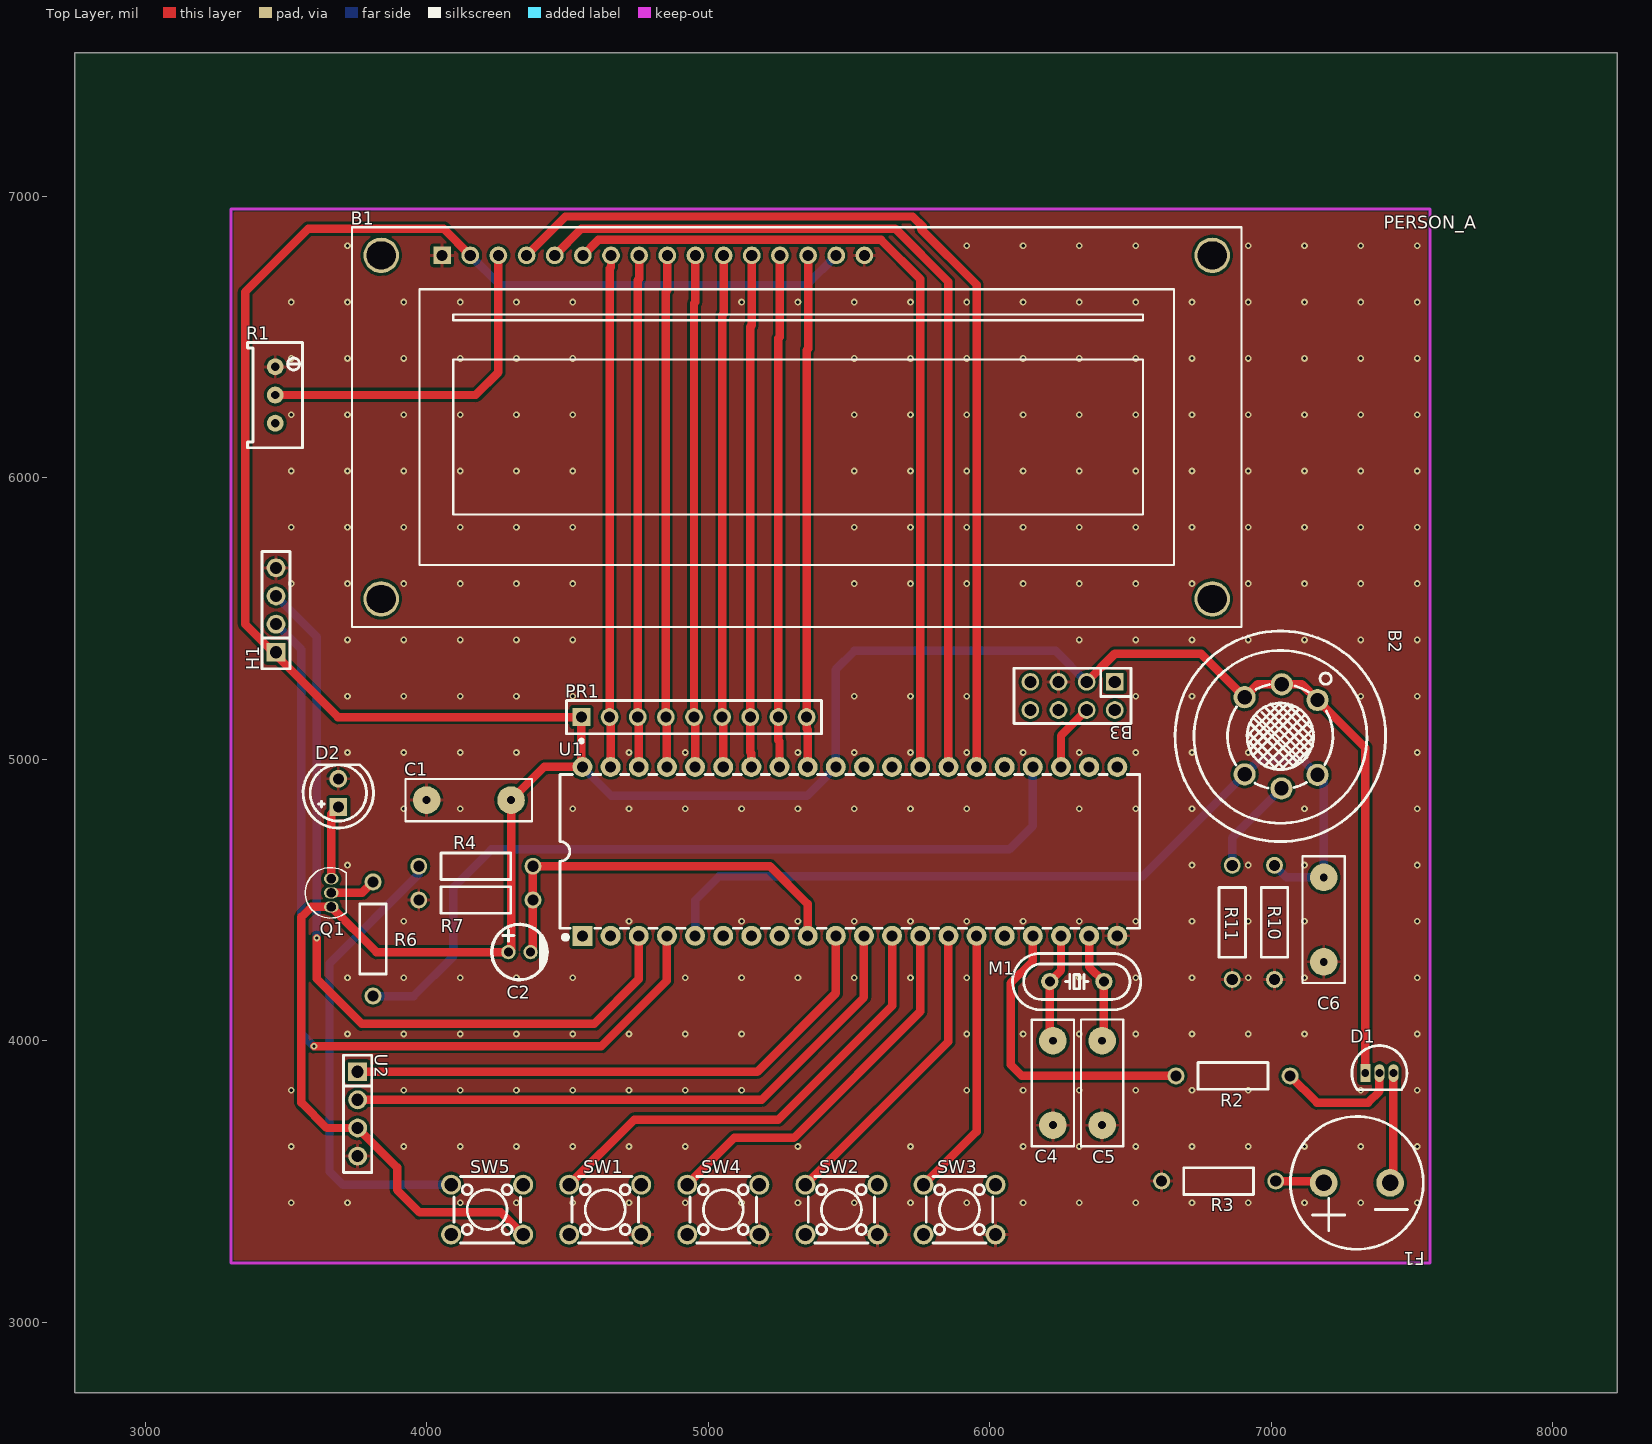
[diagram p0: Top Layer view]
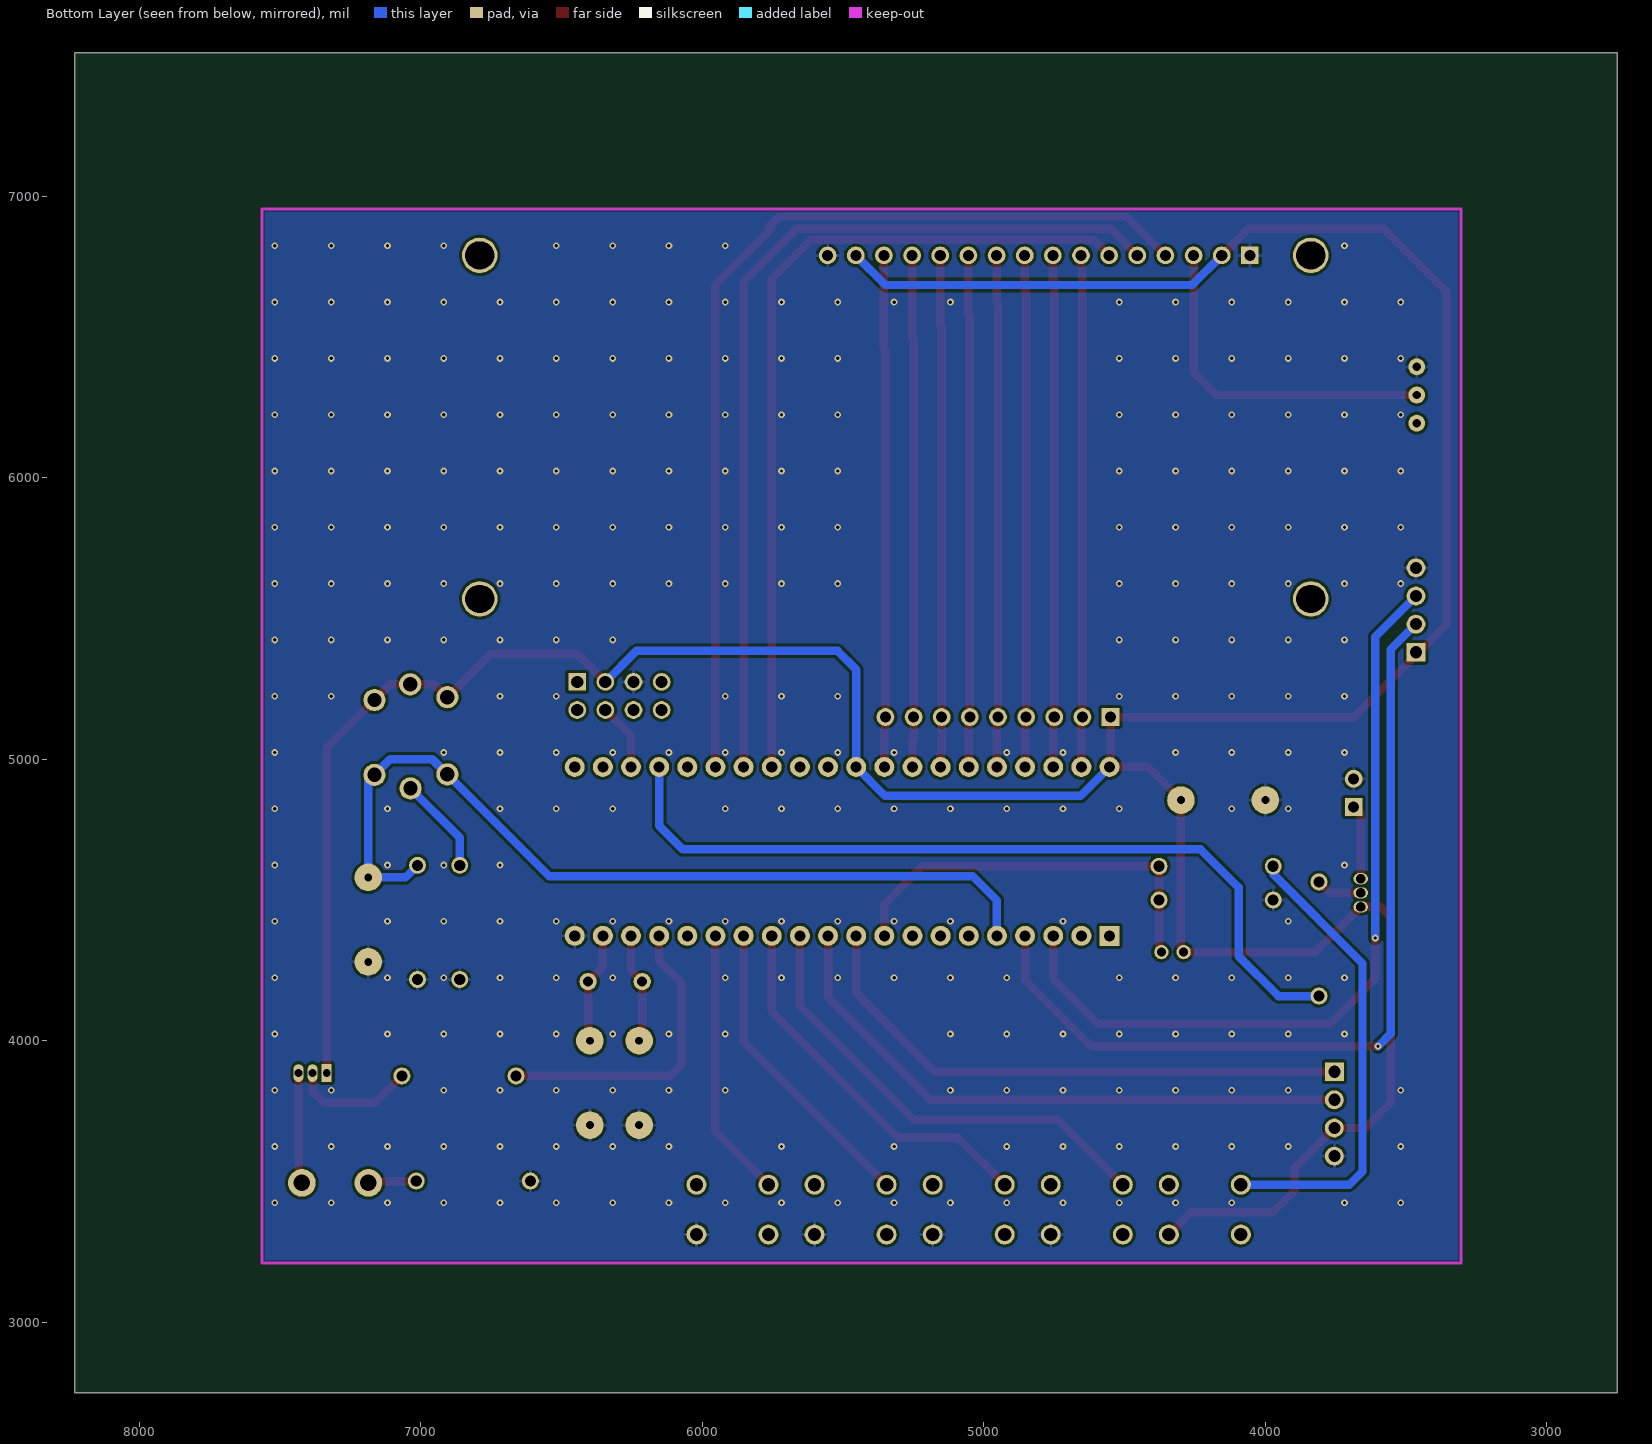
[diagram p1: Bottom Layer view, seen from below]
# Altium PCB MISC75421.pcbdoc
Units mil, origin at the board's own origin, x right, y up, seen from the top; angles counter-clockwise.
Board outline 5480 x 4760 mil, 2 copper layers (Top Layer, Bottom Layer), stack 62.206 mil thick; 30 components, 39 nets, 150 pads, 275 vias.

## Layer stack, top to bottom
Top Solder Mask Layer: solder mask 0.394, Dk 3.3
Top Layer: signal copper 1.379
Dielectric1: surface 59.449, FR4, Dk 4.5
Bottom Layer: signal copper 1.378
Bottom Solder Mask Layer: solder mask 0.394, Dk 3.3

## Board outline
8230,2750 2750,2750 2750,7510 8230,7510

## Design rules (kind name [scope] priority, off if disabled: settings)
BoardOutlineClearance copperThickness2oz_1 [All] p2 off: genericclearance=7.99 ignorepadtopadclearanceinfootprint=FALSE except(0: Arc-SplitContinuation Track-SplitContinuation SMDPad-SplitContinuation THPad-SplitContinuation Via-SplitContinuation Fill-SplitContinuation Region-SplitContinuation Poly-SplitContinuation Text-SplitContinuation Hole-SplitContinuation; 5.98: Arc-CutoutEdge SMDPad-CutoutEdge THPad-CutoutEdge Via-CutoutEdge Fill-CutoutEdge Region-CutoutEdge Text-CutoutEdge; 6.93: Hole-OutlineEdge Hole-CutoutEdge; 10: Poly-OutlineEdge Poly-CutoutEdge; 11.81: Arc-OutlineEdge Track-OutlineEdge SMDPad-OutlineEdge THPad-OutlineEdge Via-OutlineEdge Fill-OutlineEdge Region-OutlineEdge Text-OutlineEdge Track-CutoutEdge)
BoardOutlineClearance copperThickness1oz_1 [All] p4: genericclearance=4.02 ignorepadtopadclearanceinfootprint=FALSE except(0: Arc-SplitContinuation Track-SplitContinuation SMDPad-SplitContinuation THPad-SplitContinuation Via-SplitContinuation Fill-SplitContinuation Region-SplitContinuation Poly-SplitContinuation Text-SplitContinuation Hole-SplitContinuation; 6: SMDPad-CutoutEdge THPad-CutoutEdge Via-CutoutEdge Fill-CutoutEdge Region-CutoutEdge Text-CutoutEdge; 6.93: Hole-OutlineEdge Hole-CutoutEdge; 10: Poly-OutlineEdge Poly-CutoutEdge; 11.8: Arc-OutlineEdge Track-OutlineEdge SMDPad-OutlineEdge THPad-OutlineEdge Via-OutlineEdge Fill-OutlineEdge Region-OutlineEdge Text-OutlineEdge; 11.81: Arc-CutoutEdge Track-CutoutEdge)
Clearance copperThickness2oz [All] p1 off: gap=7.99 ignorepadtopadclearanceinfootprint=FALSE except(5.98: SMDPad-Track SMDPad-SMDPad THPad-Track SMDPad-THPad THPad-THPad Track-Via SMDPad-Via THPad-Via Via-Via Fill-Track Region-Track Fill-SMDPad Region-SMDPad Fill-THPad Region-THPad Fill-Via Region-Via Fill-Fill Fill-Region Region-Region Arc-Track Arc-SMDPad Arc-THPad Arc-Via Fill-Arc Region-Arc Arc-Arc Text-Track SMDPad-Text Text-THPad Text-Via Fill-Text Region-Text Arc-Text Text-Text; 6.93: Hole-Track Hole-SMDPad Hole-THPad Hole-Via Fill-Hole Region-Hole Hole-Arc Hole-Text; 10: Poly-Track Poly-SMDPad Poly-THPad Poly-Via Poly-Fill Poly-Region Poly-Poly Poly-Arc Poly-Text Poly-Hole)
Clearance copperThickness1oz [All] p3: gap=4.02 ignorepadtopadclearanceinfootprint=FALSE except(5.98: SMDPad-Track SMDPad-SMDPad THPad-Track SMDPad-THPad THPad-THPad Track-Via SMDPad-Via THPad-Via Via-Via Fill-Track Region-Track Fill-SMDPad Region-SMDPad Fill-THPad Region-THPad Fill-Via Region-Via Fill-Fill Fill-Region Region-Region; 6: Arc-Track Arc-SMDPad Arc-THPad Arc-Via Fill-Arc Region-Arc Arc-Arc Text-Track SMDPad-Text Text-THPad Text-Via Fill-Text Region-Text Arc-Text Text-Text; 6.93: Hole-Track Hole-SMDPad Hole-THPad Hole-Via Fill-Hole Region-Hole Hole-Arc Hole-Text; 10: Poly-Track Poly-SMDPad Poly-THPad Poly-Via Poly-Fill Poly-Region Poly-Poly Poly-Arc Poly-Text Poly-Hole)
DiffPairsRouting differentialPair [All] p1: maxlimit=6 minlimit=6 mostfreqgap=6 toplayer_minwidth=5 toplayer_prefwidth=10 toplayer_maxwidth=100 toplayer_mingap=6 toplayer_prefgap=6 toplayer_maxgap=6 bottomlayer_minwidth=5 bottomlayer_prefwidth=10 bottomlayer_maxwidth=100 bottomlayer_mingap=6 bottomlayer_prefgap=6 bottomlayer_maxgap=6 maxuncoupledlength=10
HoleToHoleClearance otherClearance [All] p1: gap=11.81 allowstackedmicrovias=TRUE
Length netLength [All] p1: minlimit=0 maxlimit=0
MatchedLengths netLengthTolerance [All] p1: tolerance=1000
PasteMaskExpansion pasteMaskExpansion [All] p1: expansion=0
PlaneConnect innerPlane [All] p1: planeconnectstyle=Relief reliefexpansion=20 reliefentries=4 reliefconductorwidth=10 reliefairgap=10
PolygonConnect copperRegion [(InNet('GND'))] p1: connectstyle=Relief reliefconductorwidth=10 reliefentries=4 polygonreliefangle="90 Angle" airgapwidth=10 via.connectstyle=Relief via.reliefconductorwidth=10 via.reliefentries=4 via.polygonreliefangle="90 Angle" via.airgapwidth=10
RoutingVias viaSize [All] p1: holewidth=12.01 width=24.02 viastyle="Through Hole" minholewidth=11.81 minwidth=19.68 maxholewidth=248.03 maxwidth=393.7
SolderMaskExpansion solderMaskExpansion [IsVia] p1: expansion=-1000 istentingtop=TRUE
SolderMaskExpansion solderMaskExpansion [All] p2: expansion=2 istentingtop=FALSE
Width copperThickness2oz_2 [All] p1 off: maxlimit=100 minlimit=8 preferedwidth=10
Width copperThickness1oz_2 [All] p2: maxlimit=100 minlimit=5 preferedwidth=10

## Components (designator, comment, footprint, x,y, rotation, side; value= is the part's Value field where it differs from the comment)
B1 "LCD1602" LCD1602 5315,6180 r0 top
B2 "MQ-2" SENSOR-TH_MQ-2 7035.68,5081.43 r270 top
B3 "DS18B20U+T&R" HDR-TH_8P-P2.54-V-F-R2-C4-S2.54-1 6295,5225 r180 top
C1 "Cap" RAD-0.3 4150,4855 r0 top
C2 "Electrolytic capacitor" CAP-TH_BD5.0-P2.00-D0.8-FD-10UF50VC110GL 4330,4315 r0 top
C4 "Cap" RAD-0.3 6225,3850 r90 top
C5 "Cap" RAD-0.3 6400,3850 r270 top
C6 "Cap" RAD-0.3 7187.31,4430.37 r270 top
D1 "PNP transistor" S8550P_TO-92 7385,3885 r0 top
D2 "LED0" LED-TH_5mm 3686.26,4880.55 r90 top
F1 "Buzzer" BUZ-TH_BD12.0-P6.00-D0.9-RD 7305,3495 r180 top
H1 "" HDR-TH_4P-P2.54-V-F 3465,5530 r90 top
M1 "Crystal oscillator" HC-49S_L11.5-W5.0-P4.88 6310,4210 r0 top
PR1 "8-resistor 9-pin array" RES-ARRAY-TH_9P-P2.54-D1.0 4950,5150 r0 top
Q1 "PNP" TO-92-3_L4.6-W3.6-P1.27-L_1 3661.26,4525.55 r270 top
R1 "Res Adj2" RES-ADJ-TH_3P-L9.5-W4.85-P2.54_PV36W103C01B00 3462.39,6294.12 r0 top
R2 "?K" Res_1/4W 6865,3875 r0 top
R3 "?K" Res_1/4W 6814.06,3501.48 r180 top
R4 "?K" Res_1/4W 4175,4620 r0 top
R6 "?K" Res_1/4W 3809.62,4361.5 r90 top
R7 "?K" Res_1/4W 4175,4500 r180 top
R10 "?K" Res_1/4W 7012.31,4420.37 r270 top
R11 "?K" Res_1/4W 6862.31,4420.37 r270 top
SW1 "TSW tactile switch" SW-TH_4P-L6.0-W6.0-P4.50-LS6.5 4634.57,3400 r0 top
SW2 "TSW tactile switch" SW-TH_4P-L6.0-W6.0-P4.50-LS6.5 5473.7,3400 r0 top
SW3 "TSW tactile switch" SW-TH_4P-L6.0-W6.0-P4.50-LS6.5 5893.26,3400 r0 top
SW4 "TSW tactile switch" SW-TH_4P-L6.0-W6.0-P4.50-LS6.5 5054.13,3400 r0 top
SW5 "TSW tactile switch" SW-TH_4P-L6.0-W6.0-P4.50-LS6.5 4215,3400 r180 top
U1 "STC12C5A60S2" DIP-40_L52.3-W13.9-P2.54-LS15.2-BL-BASE 5503.78,4672.72 r0 top
U2 "HC05" HDR-TH_4P-P2.54-V-F 3755,3740 r270 top

## Footprints (in the part's own frame and the unit in brackets; to place one, negate y for a bottom-side part, rotate by r counter-clockwise, add the part's x,y. Pads: shape width x height; smd on the part's side, far side on the other; paste and mask are expansions set on the pad)
BUZ-TH_BD12.0-P6.00-D0.9-RD [mm]
  round 2.5 hole 1.5 paste+0 mask+0.05: 1(-3,0) 2(3,0)
  silkscreen extent -5.99,-5.99 5.99,5.99
CAP-TH_BD5.0-P2.00-D0.8-FD-10UF50VC110GL [mm]
  round 1.3 hole 0.8: 1(-1,0) 2(1,0)
  silkscreen extent -2.5,-2.5 2.5,2.5
DIP-40_L52.3-W13.9-P2.54-LS15.2-BL-BASE [mm]
  rect 1.8x1.8 hole 1: 1(-24.13,-7.62)
  round 1.8 hole 1: 2(-21.59,-7.62) 3(-19.05,-7.62) 4(-16.51,-7.62) 5(-13.97,-7.62) 6(-11.43,-7.62) 7(-8.89,-7.62) 8(-6.35,-7.62) 9(-3.81,-7.62) 10(-1.27,-7.62) 11(1.27,-7.62) 12(3.81,-7.62) 13(6.35,-7.62) 14(8.89,-7.62) 15(11.43,-7.62) 16(13.97,-7.62) 17(16.51,-7.62) 18(19.05,-7.62) 19(21.59,-7.62) 20(24.13,-7.62) 21(24.13,7.62) 22(21.59,7.62) 23(19.05,7.62) 24(16.51,7.62) 25(13.97,7.62) 26(11.43,7.62) 27(8.89,7.62) 28(6.35,7.62) 29(3.81,7.62) 30(1.27,7.62) 31(-1.27,7.62) 32(-3.81,7.62) 33(-6.35,7.62) 34(-8.89,7.62) 35(-11.43,7.62) 36(-13.97,7.62) 37(-16.51,7.62) 38(-19.05,7.62) 39(-21.59,7.62) 40(-24.13,7.62)
  silkscreen extent -26.16,-7.95 26.16,6.93
HC-49S_L11.5-W5.0-P4.88 [mm]
  round 1.56 hole 0.9: 1(-2.44,0) 2(2.44,0)
  silkscreen extent -5.8,-2.54 5.77,2.54
HDR-TH_4P-P2.54-V-F [mm]
  rect 1.7x1.7 hole 1.1: 1(-3.81,0)
  round 1.7 hole 1.1: 2(-1.27,0) 3(1.27,0) 4(3.81,0)
  silkscreen extent -5.29,-1.27 5.29,1.27
HDR-TH_8P-P2.54-V-F-R2-C4-S2.54-1 [mm]
  rect 1.6x1.6 hole 1.1: 1(-3.81,-1.27)
  round 1.6 hole 1.1: 2(-3.81,1.27) 3(-1.27,-1.27) 4(-1.27,1.27) 5(1.27,-1.27) 6(1.27,1.27) 7(3.81,-1.27) 8(3.81,1.27)
  silkscreen extent -5.28,-2.5 5.28,2.5
LCD1602 [mm]
  round 3.2 hole 2.5 slot 2.625 at 0 deg: 0(-37.5,-15.5) 0(-37.5,15.5) 0(37.5,-15.5) 0(37.5,15.5)
  rect 1.6x1.6 hole 1: 1(-32,15.5)
  round 1.6 hole 1: 2(-29.46,15.5) 3(-26.92,15.5) 4(-24.38,15.5) 5(-21.84,15.5) 6(-19.3,15.5) 7(-16.76,15.5) 8(-14.22,15.5) 9(-11.68,15.5) 10(-9.14,15.5) 11(-6.6,15.5) 12(-4.06,15.5) 13(-1.52,15.5) 14(1.02,15.5) 15(3.56,15.5) 16(6.1,15.5)
  silkscreen extent -40.13,-18.03 40.13,18.03
LED-TH_5mm [mm]
  rect 1.6x1.6 hole 1 paste+0 mask+0.051: 1(-1.27,0)
  round 1.6 hole 1 paste+0 mask+0.051: 2(1.27,0)
  silkscreen extent -3.17,-3.17 2.54,3.17
RAD-0.3 [mil]
  round 98 hole 28: 1(150,0) 2(-150,0)
  silkscreen extent -225,-75 225,75
RES-ADJ-TH_3P-L9.5-W4.85-P2.54_PV36W103C01B00 [mil]
  round 60 hole 30: 1(0,100) 2(0,0) 3(0,-100)
  silkscreen extent -98,-187 96,187
RES-ARRAY-TH_9P-P2.54-D1.0 [mm]
  rect 1.6x1.6 hole 1: 1(-10.16,0)
  round 1.6 hole 1: 2(-7.62,0) 3(-5.08,0) 4(-2.54,0) 5(0,0) 6(2.54,0) 7(5.08,0) 8(7.62,0) 9(10.16,0)
  silkscreen extent -11.5,-2.31 11.5,1.5
Res_1/4W [mil]
  round 60 hole 39.37 paste+0 mask+2: 1(-202.76,0) 2(202.76,0)
  silkscreen extent -124,-47 124,47
S8550P_TO-92 [mm]
  rect 0.9x1.6 hole 0.7 paste+0 mask+0.051: 1(-1.27,0)
  oval 0.9x1.6 hole 0.7 paste+0 mask+0.051: 2(0,0) 3(1.27,0)
  silkscreen extent -2.48,-1.5 2.48,2.48
SENSOR-TH_MQ-2 [mil]
  round 78.74 hole 51.18: 1(-129,129.5) 2(-185,2.5) 3(-139,-129.5) 4(135,-129.5) 5(185,1.5) 6(137,129.5)
  silkscreen extent -374,-376 374,371
SW-TH_4P-L6.0-W6.0-P4.50-LS6.5 [mm]
  round 1.8 hole 1.2: 1(-3.25,2.25) 2(3.25,2.25) 3(-3.25,-2.25) 4(3.25,-2.25)
  silkscreen extent -3,-3 3,3
TO-92-3_L4.6-W3.6-P1.27-L_1 [mm]
  oval 1x1.3 hole 0.8 slot 0.84 at 90 deg paste+0 mask+0.05: 1(-1.27,0) 2(0,0) 3(1.27,0)
  silkscreen extent -2.28,-2.34 2.28,1.35

## Via types
v1: diameter 24.02, hole 12, Top Layer to Bottom Layer, 275 vias

## Nets (pads, with @x,y where several pads share a name; then routed paths per layer and width w, separated by ;. In a path a pad name is that pad's centre, name@x,y a point inside that pad or via, vN(x,y) a via of type N, cw(c..) or ccw(c..) an arc to the next point about the centre after c; other vN are vias at no path point)
$2N83: R4.1 SW5.4 | length 1667.7
  Bottom Layer w30: R4.1 3972.24,4592.24 3655,4275 3655,3535 3701.42,3488.58 SW5.4
$2N84: Q1.2 R6.2 | length 164.4
  Top Layer w30: Q1.2 3770.92,4525.55 R6.2
$2N86: B2.5 R11.1 | length 345.7
  Bottom Layer w30: R11.1 6862.31,4721.56 B2.5
$2N87: D1.2 R2.2 | length 438.2
  Top Layer w30: R2.2 7162.76,3780 7345,3780 7385,3820 D1.2
$2N88: D1.3 F1.1 | length 394.9
  Top Layer w30: F1.1 7435,3506.89 D1.3
$2N89: F1.2 R3.1 | length 172.8
  Top Layer w30: R3.1 7180.41,3501.48 F1.2
$2N91: D2.1 Q1.1 | length 265.4
  Top Layer w30: Q1.1 3661.26,4805.55 D2.1
GND: B1.1 B1.16 B3.5 C1.2 C4.2 C5.1 C6.1 D2.2 H1.4 R1.1 R3.2 R7.2 R10.2 R11.2 SW1.4 SW2.4 SW3.4 SW4.4 U1.20 U2.4
  other v1: 3519.1,3424.1 3719.1,3424.1 4119.1,3424.1 4319.1,3424.1 4519.1,3424.1 4719.1,3424.1 4919.1,3424.1 5119.1,3424.1 5319.1,3424.1 5519.1,3424.1 5719.1,3424.1 5919.1,3424.1 6119.1,3424.1 6319.1,3424.1 6519.1,3424.1 6719.1,3424.1 6919.1,3424.1 7119.1,3424.1 7319.1,3424.1 7519.1,3424.1 3519.1,3624.1 3919.1,3624.1 4119.1,3624.1 4319.1,3624.1 4519.1,3624.1 4719.1,3624.1 4919.1,3624.1 5319.1,3624.1 5719.1,3624.1 6119.1,3624.1 6319.1,3624.1 6519.1,3624.1 6719.1,3624.1 6919.1,3624.1 7119.1,3624.1 7319.1,3624.1 7519.1,3624.1 3519.1,3824.1 3919.1,3824.1 4119.1,3824.1 4319.1,3824.1 4519.1,3824.1 4719.1,3824.1 4919.1,3824.1 5119.1,3824.1 5919.1,3824.1 6119.1,3824.1 6319.1,3824.1 6519.1,3824.1 6719.1,3824.1 6919.1,3824.1 7319.1,3824.1 7519.1,3824.1 3719.1,4024.1 3919.1,4024.1 4119.1,4024.1 4319.1,4024.1 4519.1,4024.1 4719.1,4024.1 4919.1,4024.1 5119.1,4024.1 5919.1,4024.1 6119.1,4024.1 6319.1,4024.1 6519.1,4024.1 6719.1,4024.1 6919.1,4024.1 7119.1,4024.1 7519.1,4024.1 3719.1,4224.1 3919.1,4224.1 4119.1,4224.1 4319.1,4224.1 4519.1,4224.1 4919.1,4224.1 5119.1,4224.1 5319.1,4224.1 5519.1,4224.1 5719.1,4224.1 5919.1,4224.1 6319.1,4224.1 6519.1,4224.1 6719.1,4224.1 6919.1,4224.1 7119.1,4224.1 7519.1,4224.1 3919.1,4424.1 4719.1,4424.1 5119.1,4424.1 5319.1,4424.1 5519.1,4424.1 5719.1,4424.1 5919.1,4424.1 6119.1,4424.1 6319.1,4424.1 6519.1,4424.1 6719.1,4424.1 6919.1,4424.1 7119.1,4424.1 7519.1,4424.1 3719.1,4624.1 6719.1,4624.1 6919.1,4624.1 7119.1,4624.1 7519.1,4624.1 3919.1,4824.1 4119.1,4824.1 4519.1,4824.1 4719.1,4824.1 4919.1,4824.1 5119.1,4824.1 5319.1,4824.1 5519.1,4824.1 5719.1,4824.1 5919.1,4824.1 6319.1,4824.1 6519.1,4824.1 6719.1,4824.1 7119.1,4824.1 7519.1,4824.1 3719.1,5024.1 3919.1,5024.1 4119.1,5024.1 4319.1,5024.1 4719.1,5024.1 4919.1,5024.1 5319.1,5024.1 5519.1,5024.1 5719.1,5024.1 5919.1,5024.1 6119.1,5024.1 6319.1,5024.1 6519.1,5024.1 6719.1,5024.1 6919.1,5024.1 7519.1,5024.1 3719.1,5224.1 3919.1,5224.1 4119.1,5224.1 4319.1,5224.1 4519.1,5224.1 5519.1,5224.1 5719.1,5224.1 5919.1,5224.1 6519.1,5224.1 6719.1,5224.1 7319.1,5224.1 7519.1,5224.1 3719.1,5424.1 3919.1,5424.1 4119.1,5424.1 4319.1,5424.1 4519.1,5424.1 6319.1,5424.1 6519.1,5424.1 6719.1,5424.1 6919.1,5424.1 7119.1,5424.1 7319.1,5424.1 7519.1,5424.1 3519.1,5624.1 3719.1,5624.1 3919.1,5624.1 4119.1,5624.1 4319.1,5624.1 4519.1,5624.1 5519.1,5624.1 5719.1,5624.1 5919.1,5624.1 6119.1,5624.1 6319.1,5624.1 6519.1,5624.1 6719.1,5624.1 6919.1,5624.1 7119.1,5624.1 7319.1,5624.1 7519.1,5624.1 3519.1,5824.1 3719.1,5824.1 3919.1,5824.1 4119.1,5824.1 4319.1,5824.1 4519.1,5824.1 5519.1,5824.1 5719.1,5824.1 5919.1,5824.1 6119.1,5824.1 6319.1,5824.1 6519.1,5824.1 6719.1,5824.1 6919.1,5824.1 7119.1,5824.1 7319.1,5824.1 7519.1,5824.1 3519.1,6024.1 3719.1,6024.1 3919.1,6024.1 4119.1,6024.1 4319.1,6024.1 4519.1,6024.1 5519.1,6024.1 5719.1,6024.1 5919.1,6024.1 6119.1,6024.1 6319.1,6024.1 6519.1,6024.1 6719.1,6024.1 6919.1,6024.1 7119.1,6024.1 7319.1,6024.1 7519.1,6024.1 3519.1,6224.1 3719.1,6224.1 3919.1,6224.1 4119.1,6224.1 4319.1,6224.1 4519.1,6224.1 5519.1,6224.1 5719.1,6224.1 5919.1,6224.1 6119.1,6224.1 6319.1,6224.1 6519.1,6224.1 6719.1,6224.1 6919.1,6224.1 7119.1,6224.1 7319.1,6224.1 7519.1,6224.1 3519.1,6424.1 3719.1,6424.1 3919.1,6424.1 4119.1,6424.1 4319.1,6424.1 4519.1,6424.1 5519.1,6424.1 5719.1,6424.1 5919.1,6424.1 6119.1,6424.1 6319.1,6424.1 6519.1,6424.1 6719.1,6424.1 6919.1,6424.1 7119.1,6424.1 7319.1,6424.1 7519.1,6424.1 3519.1,6624.1 3719.1,6624.1 3919.1,6624.1 4119.1,6624.1 4319.1,6624.1 4519.1,6624.1 5119.1,6624.1 5319.1,6624.1 5519.1,6624.1 5719.1,6624.1 5919.1,6624.1 6119.1,6624.1 6319.1,6624.1 6519.1,6624.1 6719.1,6624.1 6919.1,6624.1 7119.1,6624.1 7319.1,6624.1 7519.1,6624.1 3719.1,6824.1 5919.1,6824.1 6119.1,6824.1 6319.1,6824.1 6519.1,6824.1 6919.1,6824.1 7119.1,6824.1 7319.1,6824.1 7519.1,6824.1
P00: B1.7 PR1.2 U1.39 | length 1821.2
  Top Layer w30: U1.39 4653.79,5146.21 PR1.2 4650,6743.58 4655.16,6748.74 B1.7
P01: B1.8 PR1.3 U1.38 | length 1821.2
  Top Layer w30: U1.38 4753.79,5146.21 PR1.3 4750,6702.16 4755.16,6707.32 B1.8
P02: B1.9 PR1.4 U1.37 | length 1821.2
  Top Layer w30: U1.37 4853.79,5146.21 PR1.4 4850,6660.74 4855.16,6665.9 B1.9
P03: B1.10 PR1.5 U1.36 | length 1821.2
  Top Layer w30: U1.36 4953.79,5146.21 PR1.5 4950,6619.32 4955.16,6624.48 B1.10
P04: B1.11 PR1.6 U1.35 | length 1821.2
  Top Layer w30: U1.35 5053.79,5146.21 PR1.6 5050,6577.9 5055.16,6583.06 B1.11
P05: B1.12 PR1.7 U1.34 | length 1821.2
  Top Layer w30: U1.34 5153.79,5021.88 5150,5025.66 PR1.7 5150,6536.48 5155.16,6541.64 B1.12
P06: B1.13 PR1.8 U1.33 | length 1821.2
  Top Layer w30: U1.33 5253.79,5063.3 5250,5067.08 PR1.8 5250,6495.06 5255.16,6500.22 B1.13
P07: B1.14 PR1.9 U1.32 | length 1821.2
  Top Layer w30: U1.32 5353.79,5104.72 5350,5108.5 PR1.9 5350,6453.63 5355.16,6458.79 B1.14
P12: H1.3 U1.3 | length 2849.8
  Top Layer w30: v1(3610,4365) 3610,4220 3770,4060 4595,4060 4753.79,4218.79 U1.3
  Bottom Layer w30: H1.3 3610,5435 v1(3610,4365)
P13: H1.2 U1.4 | length 3065.5
  Top Layer w30: v1(3600,3980) 4620,3980 4853.79,4213.79 U1.4
  Bottom Layer w30: H1.2 3555,5390 3555,4025 v1(3600,3980)
P14: B2.4 B2.6 C6.2 R10.1 U1.5 | length 3134
  Bottom Layer w30: U1.5 4953.79,4498.79 5040,4585 6544.75,4585 B2.4 6959.75,5000 7109.6,5000 B2.6 7187.31,4922.29 C6.2 7055.07,4580.37 R10.1
P20: U1.21
P21: U1.22
P22: B3.4 U1.23 | length 240.1
  Top Layer w30: U1.23 6253.79,5083.79 B3.4
P23: R6.1 U1.24 | length 2947.2
  Bottom Layer w30: R6.1 3953.74,4158.74 4095,4300 4095,4545 4230,4680 6070,4680 6153.79,4763.79 U1.24
P25: B1.4 U1.26 | length 3473.9
  Top Layer w30: B1.4 4493.12,6928.2 5726.8,6928.2 5765,6890 ; 5757.5,6882.5 5953.79,6686.21 U1.26
P26: B1.5 U1.27 | length 3239.6
  Top Layer w30: B1.5 4549.92,6885 5665,6885 5853.79,6696.21 U1.27
P27: B1.6 U1.28 | length 3012.3
  Top Layer w30: B1.6 4609.92,6845 5615,6845 5753.79,6706.21 U1.28
P32: SW1.1 U1.12 | length 1659.2
  Top Layer w30: SW1.1 4738.04,3720 5250,3720 5653.79,4123.79 U1.12
P33: SW4.1 U1.13 | length 1351.4
  Top Layer w30: SW4.1 5092.6,3655 5305,3655 5753.79,4103.79 U1.13
P34: SW2.1 U1.14 | length 1094.6
  Top Layer w30: SW2.1 5853.79,3996.62 U1.14
P35: SW3.1 U1.15 | length 962.2
  Top Layer w30: SW3.1 5953.79,3677.05 U1.15
P36: U1.16
P37: R2.1 U1.17 | length 1094.2
  Top Layer w30: U1.17 6153.79,4283.79 6075,4205 6075,3915 6115,3875 R2.1
RES: C2.2 R4.2 R7.1 U1.9 | length 1453.4
  Top Layer w30: C2.2 4377.76,4323.39 R7.1 R4.2 5220,4620 5353.79,4486.21 U1.9
RXD: U1.10 U2.1 | length 2018.2
  Top Layer w30: U2.1 5175,3890 5453.79,4168.79 U1.10
TXD: U1.11 U2.2 | length 2168.4
  Top Layer w30: U2.2 5190,3790 5553.79,4153.79 U1.11
VCC: B1.2 B1.15 B2.1 B2.2 B2.3 B3.3 C1.1 C2.1 D1.1 H1.1 PR1.1 Q1.3 SW5.1 U1.31 U1.40 U2.3 | length 13021.5
  Top Layer w30: B1.2 4060.4,6885 3580,6885 3355,6660 3355,5480 3685,5150 PR1.1 4550,4976.5 U1.40 4417.72,4972.72 C1.1 4300,4324.37 C2.1 3821.81,4315 Q1.3 3590.55,4475.55 3555,4440 3555,3780 3645,3690 U2.3 3895,3550 3895,3470 3975,3390 4264.37,3390 SW5.1 ; B3.3 6445,5375 6751.6,5375 B2.3 6952.18,5266.43 B2.2 7109.18,5266.43 B2.1 7335,5040.6 D1.1
  Bottom Layer w30: B1.2 4260.4,6685 5349.92,6685 B1.15 ; U1.40 4656.5,4870 5351.07,4870 U1.31 5453.79,5318.79 5520,5385 6235,5385 B3.3
VEE: B1.3 R1.2 | length 1241.4
  Top Layer w30: R1.2 4174.11,6294.11 4255.16,6375.16 B1.3
XTAL1: C5.2 M1.2 U1.19 | length 396.9
  Top Layer w30: U1.19 6353.79,4262.27 M1.2 6406.06,4006.06 C5.2
XTAL2: C4.1 M1.1 U1.18 | length 393.8
  Top Layer w30: C4.1 6213.94,4011.06 M1.1 6253.79,4249.85 U1.18
pads on no net: B1.0 B3.1 B3.2 B3.6 B3.7 B3.8 R1.3 SW1.2 SW1.3 SW2.2 SW2.3 SW3.2 SW3.3 SW4.2 SW4.3 SW5.2 SW5.3 U1.1 U1.2 U1.6 U1.7 U1.8 U1.25 U1.29 U1.30

## Polygon pours and split planes (outlines as drawn)
GND on Bottom Layer (solid, remove dead copper, pour order 2): 3000,7260 3000,3000 7980,3000 7980,7260
GND on Top Layer (solid, remove dead copper, pour order 0): 3170,7070 3170,3030 7870,3030 7870,7070

## Keep-outs
Board Outline Layer:
  lines w10: 3305,3210 3305,6955 7565,6955 7565,3210 3305,3210

## Silkscreen, mask and mechanical layers (free items; w line width, h text height)
Top Silkscreen Layer:
  text "PERSON_A" at 7400,6885 h45